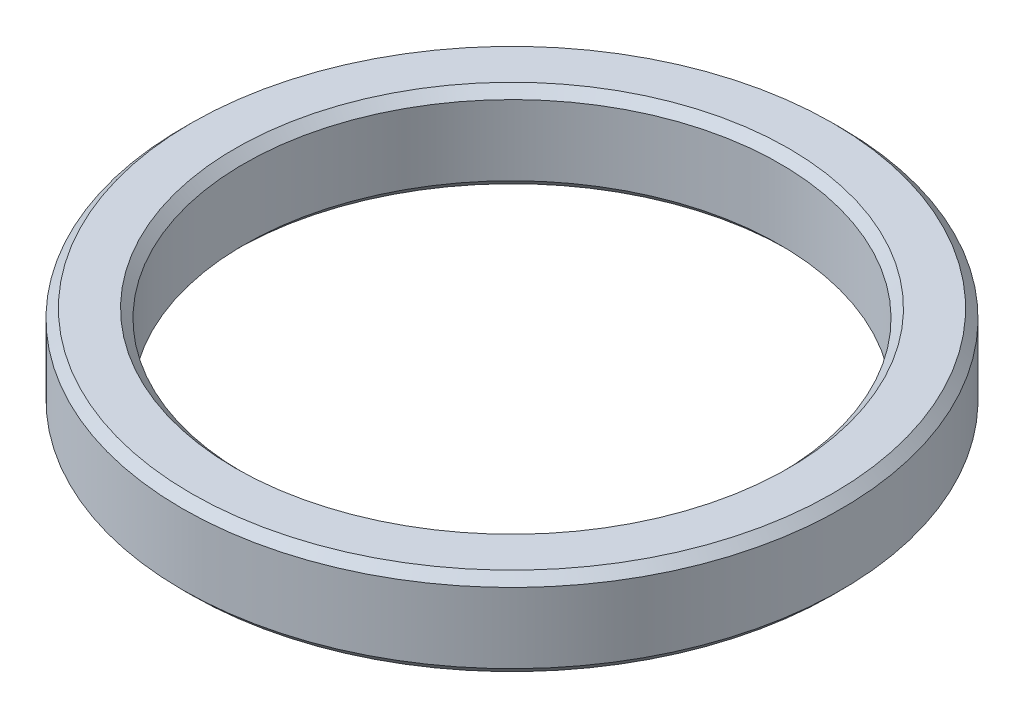
from build123d import *

# Parameters (mm, degrees)
SKETCH1_R           = 37.5
SKETCH1_R_2         = 30.5
BOSS_EXTRUDE1_DEPTH = 10
CHAMFER1_SIZE       = 1


with BuildPart() as part:
    # Sketch1 → Boss-Extrude1 (new body)
    with BuildSketch(Plane(origin=(0, 0, 0), x_dir=(1, 0, 0), z_dir=(0, 1, 0))):
        with Locations(Location((0, 0, 0), (0, 0, 270))):
            Circle(SKETCH1_R)
        with Locations(Location((0, 0, 0), (0, 0, 270))):
            Circle(SKETCH1_R_2, mode=Mode.SUBTRACT)
    extrude(amount=BOSS_EXTRUDE1_DEPTH)

    # Chamfer1
    chamfer1_edges = [part.edges().sort_by_distance(p)[0] for p in [
        (0, 0, -37.5),
        (0, 10, -37.5),
        (0, 0, -30.5),
        (0, 10, -30.5),
    ]]
    chamfer(chamfer1_edges, length=CHAMFER1_SIZE)


solid = part.part
